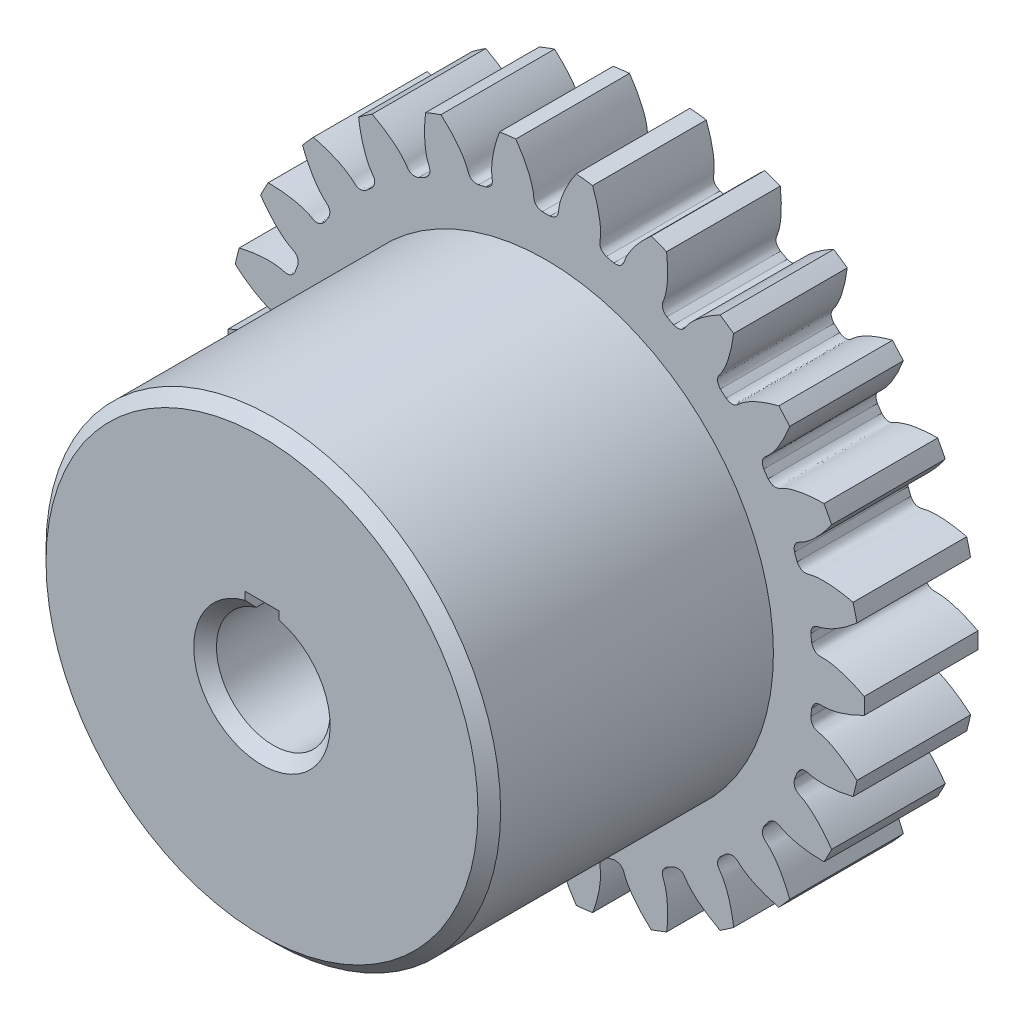
from build123d import *

# Parameters (mm, degrees)
SKETCH1_R           = 28
BOSS_EXTRUDE1_DEPTH = 10
CUT_EXTRUDE1_DEPTH  = 41.841155713
CIRPATTERN1_COUNT   = 26
SKETCH9_R           = 20
BOSS_EXTRUDE3_DEPTH = 25
SKETCH10_R          = 5
CUT_EXTRUDE5_DEPTH  = 35
CHAMFER2_SIZE       = 1
SKETCH11_W          = 3
SKETCH11_H          = 3
CUT_EXTRUDE6_DEPTH  = 35


with BuildPart() as part:
    # Sketch1 → Boss-Extrude1 (new body)
    with BuildSketch(Plane.XY):
        Circle(SKETCH1_R)
    extrude(amount=BOSS_EXTRUDE1_DEPTH)

    # Sketch2 → Cut-Extrude1 (cut, through all)
    with BuildSketch(Plane.XY):
        with BuildLine():
            ThreePointArc((0.334166203, 23.497623985), (0, 23.5), (-0.334166203, 23.497623985))
            add(Edge.make_bspline(
                [(-0.334166203, 23.497623985), (-1.126249154, 23.647573059), (-1.060682993, 24.115894486), (-1.134806649, 24.58436917), (-1.145940464, 24.646912416), (-1.160233381, 24.718805072), (-1.178047812, 24.799945437), (-1.199763487, 24.890216464), (-1.225750213, 24.989491134), (-1.256376305, 25.097630828), (-1.292005509, 25.214485967), (-1.332997575, 25.339895945), (-1.379707694, 25.473689291), (-1.432486291, 25.615683768), (-1.491678707, 25.765686504), (-1.557624929, 25.923494124), (-1.6306593, 26.088892886), (-1.711110243, 26.261658827), (-1.79929999, 26.441557916), (-1.895544305, 26.628346218), (-2.000152224, 26.821770052), (-2.113425787, 27.02156617), (-2.235659783, 27.227461935), (-2.367141495, 27.439175509), (-2.508150449, 27.656416042), (-2.658958171, 27.878883872), (-2.819827949, 28.106270733), (-2.991014594, 28.338259962), (-3.172764214, 28.574526716), (-3.365313988, 28.8147382), (-3.568891947, 29.058553888), (-3.783716762, 29.305625763), (-4.009997535, 29.555598554), (-4.2479336, 29.80810998), (-4.497714323, 30.062791), (-4.759518919, 30.31926607), (-5.033516256, 30.5771534), (-5.31986471, 30.836065219), (-5.618711894, 31.095608048), (-6.039026251, 31.446147682), (-6.365991342, 31.702419987), (-6.589818312, 31.870903728)],
                knots=[0, 0, 0, 0, 0.122665365, 0.127715434, 0.133683697, 0.140570154, 0.148374806, 0.157097651, 0.166738691, 0.177297926, 0.188775354, 0.201170977, 0.214484794, 0.228716806, 0.243867011, 0.259935411, 0.276922005, 0.294826794, 0.313649777, 0.333390954, 0.354050325, 0.37562789, 0.39812365, 0.421537604, 0.445869753, 0.471120096, 0.497288632, 0.524375364, 0.552380289, 0.581303409, 0.611144723, 0.641904231, 0.673581934, 0.706177831, 0.739691922, 0.774124208, 0.809474687, 0.845743361, 0.88293023, 0.921035292, 1, 1, 1, 1], degree=3))
            ThreePointArc((-6.589818312, 31.870903728), (0, 32.54504893), (6.589818312, 31.870903728))
            add(Edge.make_bspline(
                [(0.334166203, 23.497623985), (1.126249154, 23.647573059), (1.060682993, 24.115894486), (1.134806649, 24.58436917), (1.145940464, 24.646912416), (1.160233381, 24.718805072), (1.178047812, 24.799945437), (1.199763487, 24.890216464), (1.225750213, 24.989491134), (1.256376305, 25.097630828), (1.292005509, 25.214485967), (1.332997575, 25.339895945), (1.379707694, 25.473689291), (1.432486291, 25.615683768), (1.491678707, 25.765686504), (1.557624929, 25.923494124), (1.6306593, 26.088892886), (1.711110243, 26.261658827), (1.79929999, 26.441557916), (1.895544305, 26.628346218), (2.000152224, 26.821770052), (2.113425787, 27.02156617), (2.235659783, 27.227461935), (2.367141495, 27.439175509), (2.508150449, 27.656416042), (2.658958171, 27.878883872), (2.819827949, 28.106270733), (2.991014594, 28.338259962), (3.172764214, 28.574526716), (3.365313988, 28.8147382), (3.568891947, 29.058553888), (3.783716762, 29.305625763), (4.009997535, 29.555598554), (4.2479336, 29.80810998), (4.497714323, 30.062791), (4.759518919, 30.31926607), (5.033516256, 30.5771534), (5.31986471, 30.836065219), (5.618711894, 31.095608048), (6.039026251, 31.446147682), (6.365991342, 31.702419987), (6.589818312, 31.870903728)],
                knots=[0, 0, 0, 0, 0.122665365, 0.127715434, 0.133683697, 0.140570154, 0.148374806, 0.157097651, 0.166738691, 0.177297926, 0.188775354, 0.201170977, 0.214484794, 0.228716806, 0.243867011, 0.259935411, 0.276922005, 0.294826794, 0.313649777, 0.333390954, 0.354050325, 0.37562789, 0.39812365, 0.421537604, 0.445869753, 0.471120096, 0.497288632, 0.524375364, 0.552380289, 0.581303409, 0.611144723, 0.641904231, 0.673581934, 0.706177831, 0.739691922, 0.774124208, 0.809474687, 0.845743361, 0.88293023, 0.921035292, 1, 1, 1, 1], degree=3))
        make_face()
    cut_extrude1 = extrude(amount=CUT_EXTRUDE1_DEPTH, mode=Mode.SUBTRACT)

    # CirPattern1: Cut-Extrude1 ×26 about axis
    cirpattern1_axis = Axis((0, 0, -0.5), (0, 0, 1))
    for i in range(1, CIRPATTERN1_COUNT):
        add(cut_extrude1.rotate(cirpattern1_axis, i * 360 / CIRPATTERN1_COUNT), mode=Mode.SUBTRACT)

    # Sketch9 → Boss-Extrude3 (add)
    with BuildSketch(Plane.XY.offset(10)):
        Circle(SKETCH9_R)
    extrude(amount=BOSS_EXTRUDE3_DEPTH)

    # Sketch10 → Cut-Extrude5 (cut)
    with BuildSketch(Plane.XY.offset(35)):
        Circle(SKETCH10_R)
    extrude(amount=-CUT_EXTRUDE5_DEPTH, mode=Mode.SUBTRACT)

    # Chamfer2
    chamfer2_edges = [part.edges().sort_by_distance(p)[0] for p in [
        (-20, 0, 35),
        (-5, 0, 0),
        (-5, 0, 35),
    ]]
    chamfer(chamfer2_edges, length=CHAMFER2_SIZE)

    # Sketch11 → Cut-Extrude6 (cut)
    with BuildSketch(Plane.XY.offset(35)):
        with Locations((0, 5)):
            Rectangle(SKETCH11_W, SKETCH11_H)
    extrude(amount=-CUT_EXTRUDE6_DEPTH, mode=Mode.SUBTRACT)


solid = part.part
